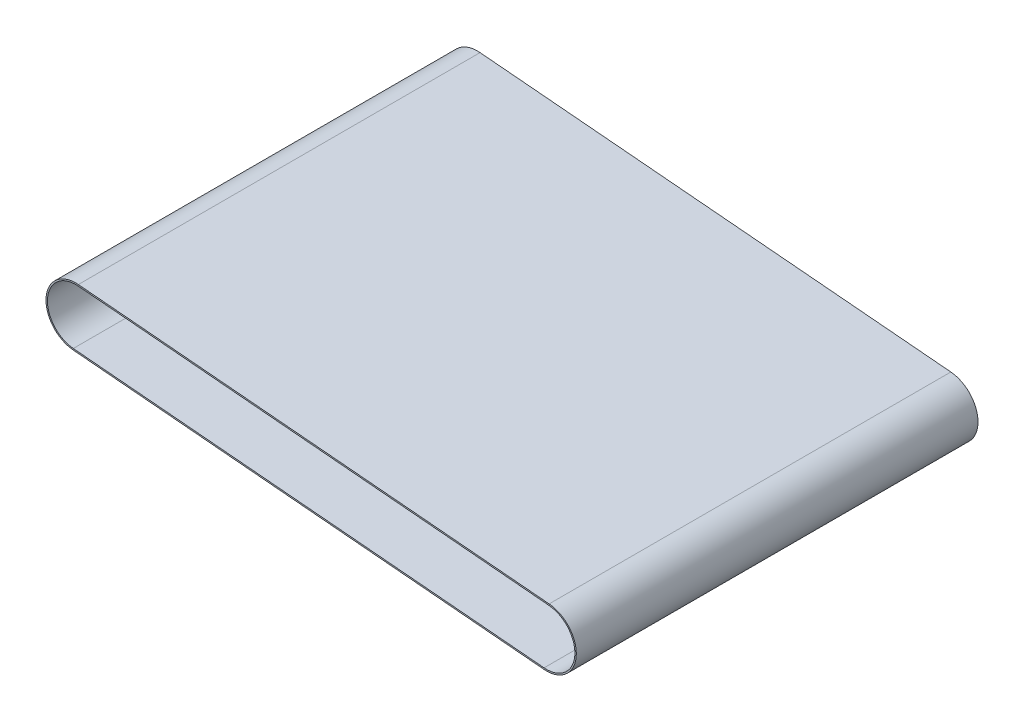
from build123d import *

# Parameters (mm, degrees)
EXTRUDE_1_DEPTH = 850


with BuildPart() as part:
    # 草图1 → 凸台-拉伸1 (new body)
    with BuildSketch(Plane.XY.offset(425)):
        with BuildLine():
            Line((2520.186202106, 858.855453105), (3516.380900198, 771.699710358))
            ThreePointArc((3516.380900198, 771.699710358), (3573.650354384, 703.448632585), (3505.399276611, 646.179178398))
            Line((3505.399276611, 646.179178398), (2509.20457852, 733.334921146))
            ThreePointArc((2509.20457852, 733.334921146), (2451.935124333, 801.585998919), (2520.186202106, 858.855453105))
        make_face()
        with BuildLine():
            Line((2519.924734878, 855.866869011), (3516.119432969, 768.711126263))
            ThreePointArc((3516.119432969, 768.711126263), (3570.66177029, 703.710099813), (3505.66074384, 649.167762492))
            Line((3505.66074384, 649.167762492), (2509.466045748, 736.32350524))
            ThreePointArc((2509.466045748, 736.32350524), (2454.923708427, 801.32453169), (2519.924734878, 855.866869011))
        make_face(mode=Mode.SUBTRACT)
    extrude(amount=-EXTRUDE_1_DEPTH)


solid = part.part
